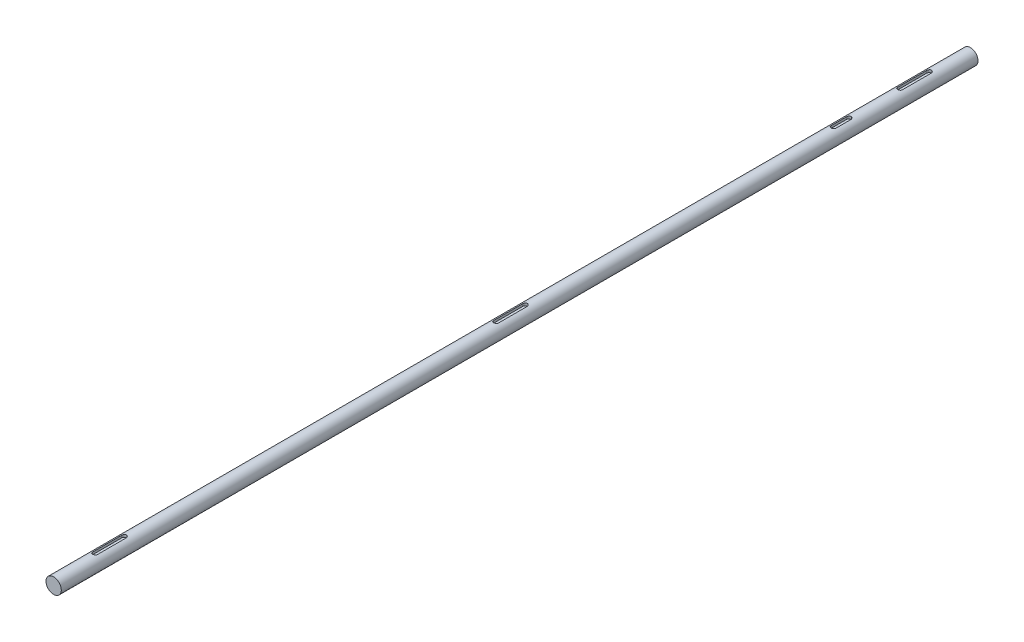
from build123d import *

# Parameters (mm, degrees)
SKETCH_1_R          = 10
EXTRUDE_1_DEPTH     = 599
CUT_EXTRUDE_START   = 10
CUT_EXTRUDE_3_DEPTH = 3.5


with BuildPart() as part:
    # 草图1 → 凸台-拉伸1 (new, symmetric)
    with BuildSketch(Plane.XY):
        Circle(SKETCH_1_R)
    extrude(amount=EXTRUDE_1_DEPTH, both=True)

    # 草图3 → 切除-拉伸3 (cut)
    with BuildSketch(Plane(origin=(0, 0, 0), x_dir=(1, 0, 0), z_dir=(0, 1, 0)).offset(CUT_EXTRUDE_START)):
        with BuildLine():
            Line((-3, 507), (-3, 545))
            ThreePointArc((-3, 545), (0, 548), (3, 545))
            Line((3, 545), (3, 507))
            ThreePointArc((3, 507), (0, 504), (-3, 507))
        make_face()
        with BuildLine():
            Line((-3, -507), (-3, -545))
            ThreePointArc((-3, -545), (0, -548), (3, -545))
            Line((3, -545), (3, -507))
            ThreePointArc((3, -507), (0, -504), (-3, -507))
        make_face()
        with BuildLine():
            Line((3, 440), (3, 420))
            ThreePointArc((3, 420), (0, 417), (-3, 420))
            Line((-3, 420), (-3, 440))
            ThreePointArc((-3, 440), (0, 443), (3, 440))
        make_face()
        with BuildLine():
            Line((-3, -21), (-3, 17))
            ThreePointArc((-3, 17), (0, 20), (3, 17))
            Line((3, 17), (3, -21))
            ThreePointArc((3, -21), (0, -24), (-3, -21))
        make_face()
    extrude(amount=-CUT_EXTRUDE_3_DEPTH, mode=Mode.SUBTRACT)


solid = part.part
